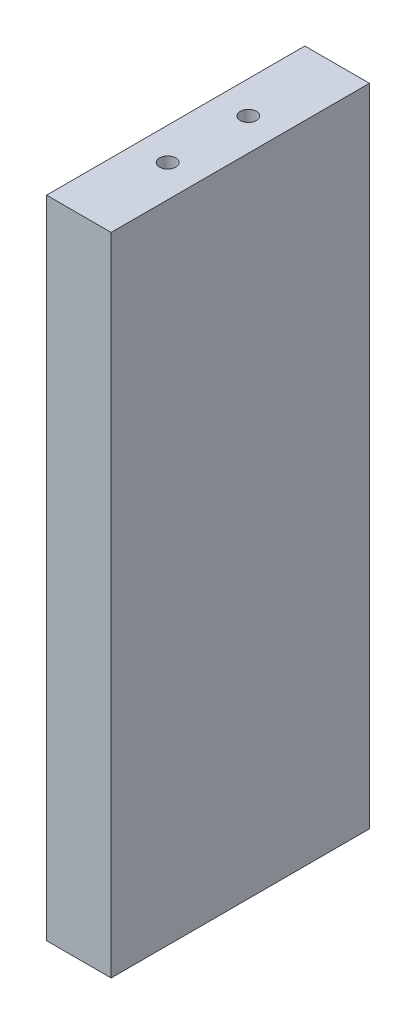
SolidWorks part; units mm, degrees
ref_plane "前视基准面" through (0, 0, 0) normal (0, 0, 1) x (1, 0, 0)
ref_plane "上视基准面" through (0, 0, 0) normal (0, 1, 0) x (1, 0, 0)
ref_plane "右视基准面" through (0, 0, 0) normal (1, 0, 0) x (0, 0, -1)
sketch "草图1" plane through (0, 0, 0) normal (1, 0, 0) x (0, 0, -1)
  line L1 (-40, 100) -> (40, 100)
  line L2 (-40, 100) -> (-40, -100)
  line L3 (-40, -100) -> (40, -100)
  line L4 (40, 100) -> (40, -100)
  line L5 (-40, 100) -> (40, -100) construction
  line L6 (-40, -100) -> (40, 100) construction
  point P0 (0, 0)
  dimension "D1" = 80
  dimension "D2" = 200
extrude "凸台-拉伸1" add sketch "草图1" along normal blind 20
hole_wizard "M6 螺纹孔1" positions "草图2" profile "草图3" tap size "M6" standard "GB"
sketch "草图2" plane through (0, 100, 0) normal (0, 1, 0) x (1, 0, 0)
  line L0 (10, -40) -> (10, 107.5325) construction
  line L1 (20, -40) -> (0, -40) construction
  line L3 (0, 0) -> (40.3433, 0) construction
  point P0 (10, 12.5)
  point P4 (10, -12.5)
  dimension "D1" = 25
sketch "草图3" plane through (10, 100, -12.5) normal (1, 0, 0) x (0, 0, 1)
  line L0 (0, 0) -> (0, 21.5022)
  line L1 (0, 21.5022) -> (2.5, 20)
  line L2 (2.5, 20) -> (2.5, 0)
  line L5 (2.5, 0) -> (0, 0)
  line L10 (0, 21.5022) -> (-2.5, 20) construction
  line L11 (0, -6.35) -> (0, 107.95) construction
  dimension "螺纹孔钻头直径" = 5
  dimension "螺纹孔钻头深度" = 20
  dimension "导头角度" = 118
cosmetic thread "孔螺蚊线1"
cosmetic thread "孔螺蚊线3"
hole_wizard "M6 螺纹孔2" positions "草图4" profile "草图5" tap size "M6" standard "GB"
sketch "草图4" plane through (0, -100, 0) normal (0, -1, 0) x (-1, 0, 0)
  line L0 (0, 0) -> (-36.9251, 0) construction
  line L2 (-10, -40) -> (-10, -7.0649) construction
  line L3 (-20, -40) -> (0, -40) construction
  point P0 (-10, 20)
  point P2 (-10, -20)
  dimension "D1" = 40
sketch "草图5" plane through (10, -100, -20) normal (1, 0, 0) x (0, 0, -1)
  line L0 (0, 0) -> (0, 24.5022)
  line L1 (0, 24.5022) -> (2.5, 23)
  line L2 (2.5, 23) -> (2.5, 0)
  line L5 (2.5, 0) -> (0, 0)
  line L10 (0, 24.5022) -> (-2.5, 23) construction
  line L11 (0, -6.35) -> (0, 107.95) construction
  dimension "螺纹孔钻头直径" = 5
  dimension "螺纹孔钻头深度" = 23
  dimension "导头角度" = 118
cosmetic thread "孔螺蚊线4"
cosmetic thread "孔螺蚊线5"
